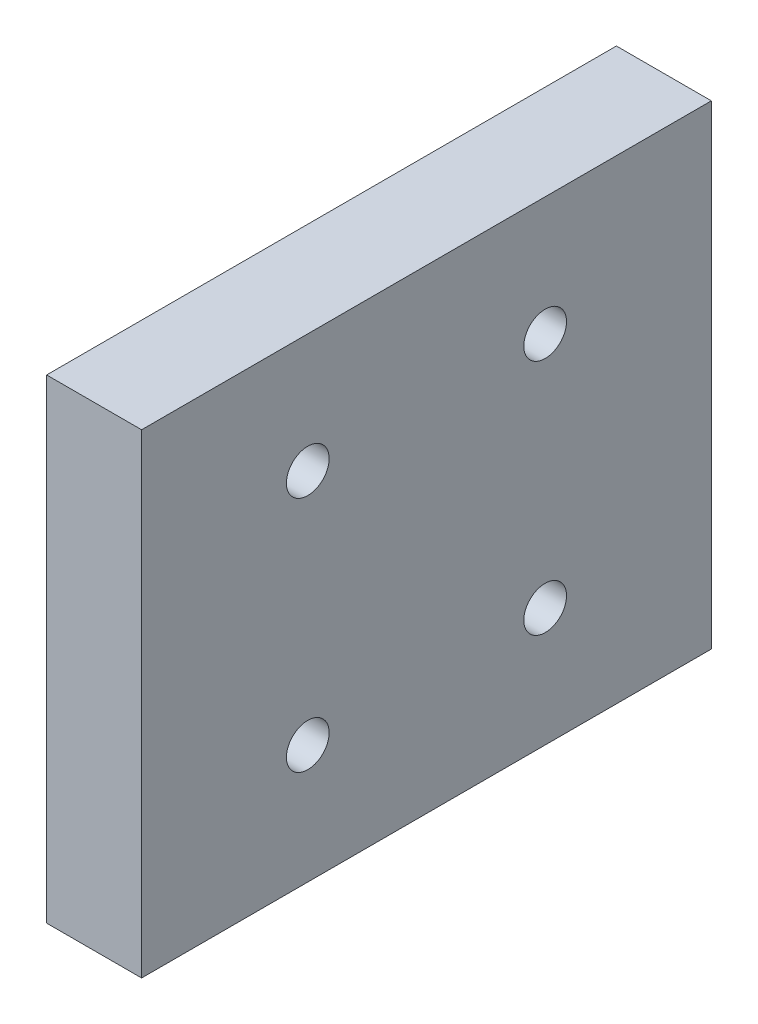
SolidWorks part; units mm, degrees
ref_plane "前视基准面" through (0, 0, 0) normal (0, 0, 1) x (1, 0, 0)
ref_plane "上视基准面" through (0, 0, 0) normal (0, 1, 0) x (1, 0, 0)
ref_plane "右视基准面" through (0, 0, 0) normal (1, 0, 0) x (0, 0, -1)
sketch "草图1" plane through (0, 0, 0) normal (1, 0, 0) x (0, 0, -1)
  line L1 (-60, 50) -> (60, 50)
  line L2 (-60, 50) -> (-60, -50)
  line L3 (-60, -50) -> (60, -50)
  line L4 (60, 50) -> (60, -50)
  line L5 (-60, 50) -> (60, -50) construction
  line L6 (-60, -50) -> (60, 50) construction
  point P0 (0, 0)
  dimension "D1" = 120
  dimension "D2" = 100
extrude "凸台-拉伸1" add sketch "草图1" along normal blind 20
hole_wizard "Ø9.0 (9) 直径孔1" positions "草图2" profile "草图3" hole size "Ø9.0" standard "GB" end condition through all
sketch "草图2" plane through (20, 0, 0) normal (1, 0, 0) x (0, 0, -1)
  line L0 (0, 60.9926) -> (0, 0) construction
  line L1 (0, 0) -> (64.2803, 0) construction
  point P0 (-25, 25)
  point P2 (25, 25)
  point P4 (-25, -25)
  point P6 (25, -25)
  dimension "D1" = 50
  dimension "D2" = 50
sketch "草图3" plane through (20, 25, 25) normal (0, 1, 0) x (0, 0, -1)
  line L0 (0, 0) -> (0, 20)
  line L1 (0, 20) -> (4.5, 20)
  line L2 (4.5, 20) -> (4.5, 0)
  line L5 (4.5, 0) -> (0, 0)
  line L11 (0, -6.35) -> (0, 107.95) construction
  dimension "通孔孔直径" = 9
  dimension "通孔孔深度" = 20
